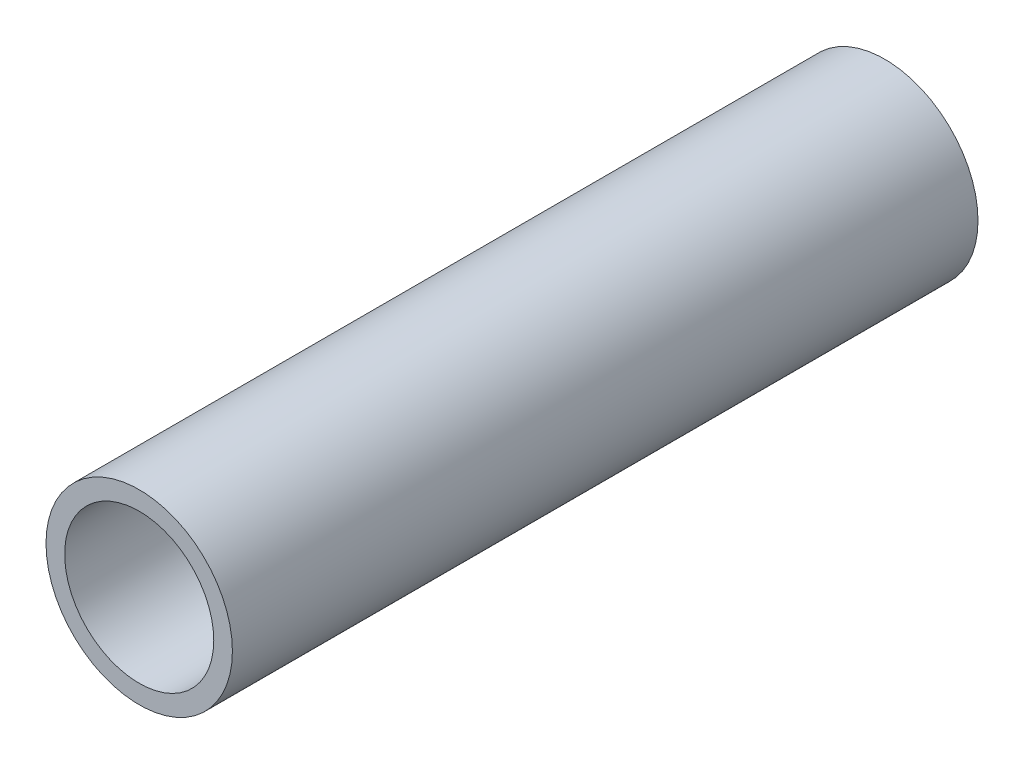
from build123d import *

# Parameters (mm, degrees)
SKETCH_1_R      = 25
SKETCH_1_R_2    = 20
EXTRUDE_1_DEPTH = 200


with BuildPart() as part:
    # 草图1 → 凸台-拉伸1 (new body)
    with BuildSketch(Plane.XY):
        Circle(SKETCH_1_R)
        Circle(SKETCH_1_R_2, mode=Mode.SUBTRACT)
    extrude(amount=EXTRUDE_1_DEPTH)


solid = part.part
